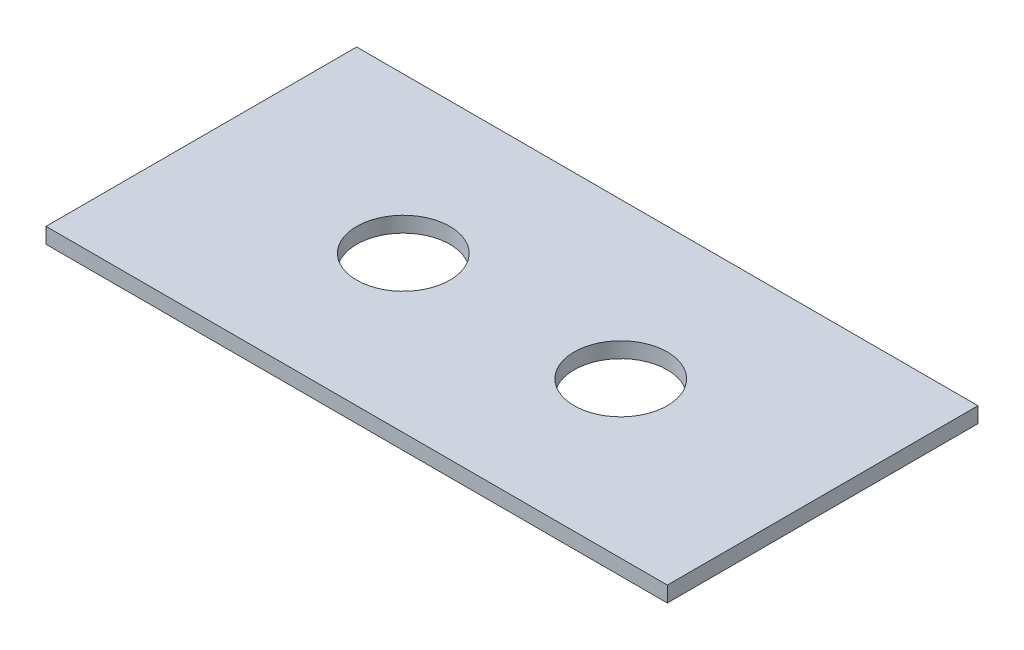
SolidWorks part; units mm, degrees
material "铜H591"
ref_plane "Front Plane" through (0, 0, 0) normal (0, 0, 1) x (1, 0, 0)
ref_plane "Top Plane" through (0, 0, 0) normal (0, 1, 0) x (1, 0, 0)
ref_plane "Right Plane" through (0, 0, 0) normal (1, 0, 0) x (0, 0, -1)
sketch "Sketch1" plane through (0, 0, 0) normal (0, 1, 0) x (1, 0, 0)
  line L0 (0, 5) -> (0, -5) construction
  line L1 (-10, -5) -> (10, -5)
  line L2 (-10, -5) -> (-10, 5)
  line L3 (-10, 5) -> (10, 5)
  line L4 (10, -5) -> (10, 5)
  line L5 (-10, -5) -> (10, 5) construction
  line L6 (-10, 5) -> (10, -5) construction
  circle A0 centre (-3.5, 0) radius 1.5
  circle A1 centre (3.5, 0) radius 1.5
  point P0 (0, 0)
  dimension "D3" = 3
  dimension "D1" = 10
  dimension "D2" = 20
  dimension "D4" = 7
extrude "Boss-Extrude1" add sketch "Sketch1" along normal blind 0.5
